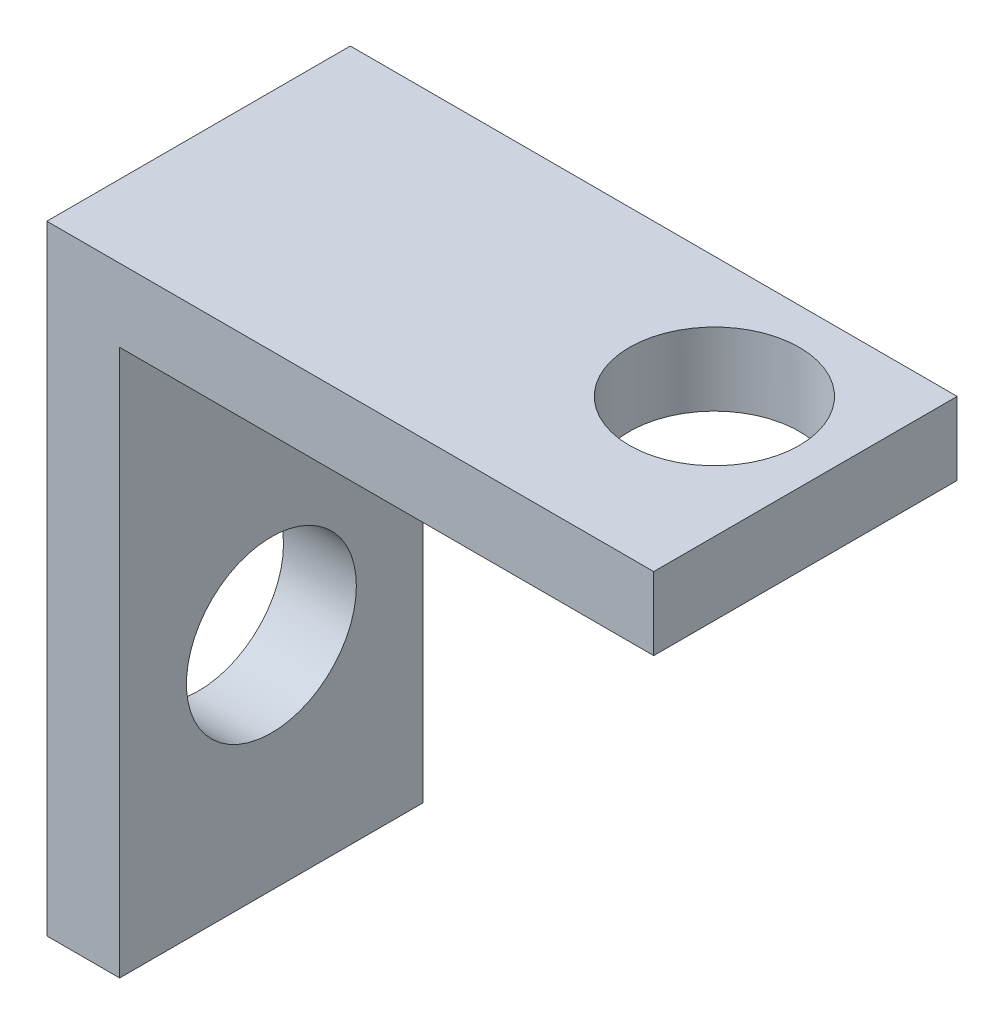
from build123d import *

# Parameters (mm, degrees)
SKETCH1_W               = 40
SKETCH1_H               = 50
BOSS_EXTRUDE1_DEPTH     = 12
CUT_EXTRUDE1_DEPTH      = 35.190641995
CUT_EXTRUDE1_DEPTH_BACK = 35.190641995
SKETCH2_R               = 14
MOVE_FACE2_BY           = 60
SKETCH3_W               = 12
SKETCH3_H               = 50
BOSS_EXTRUDE2_DEPTH     = 90
CUT_EXTRUDE2_DEPTH      = 129.33160172
CUT_EXTRUDE2_DEPTH_BACK = 129.33160172
SKETCH4_R               = 14


with BuildPart() as part:
    # Sketch1 → Boss-Extrude1 (new body)
    with BuildSketch(Plane(origin=(0, 0, 0), x_dir=(1, 0, 0), z_dir=(0, 1, 0))):
        Rectangle(SKETCH1_W, SKETCH1_H)
    extrude(amount=BOSS_EXTRUDE1_DEPTH)

    # Sketch2 → Cut-Extrude1 (cut, two sides: drawn at the far end of the back side and taken through both)
    with BuildSketch(Plane(origin=(0, 12, 0), x_dir=(1, 0, 0), z_dir=(0, 1, 0)).offset(-CUT_EXTRUDE1_DEPTH_BACK)):
        with Locations(Location((0, 5, 0), (0, 0, 270))):
            Circle(SKETCH2_R)
    extrude(amount=CUT_EXTRUDE1_DEPTH + CUT_EXTRUDE1_DEPTH_BACK, mode=Mode.SUBTRACT)

    # Move Face2: a face moved outward by 60.0
    extrude(part.faces().sort_by_distance((-20, 6, 0))[0], amount=MOVE_FACE2_BY, dir=(-1, 0, 0))

    # Sketch3 → Boss-Extrude2 (add)
    with BuildSketch(Plane(origin=(0, 0, 0), x_dir=(1, 0, 0), z_dir=(0, 1, 0))):
        with Locations((-74, 0)):
            Rectangle(SKETCH3_W, SKETCH3_H)
    extrude(amount=-BOSS_EXTRUDE2_DEPTH)

    # Sketch4 → Cut-Extrude2 (cut, two sides: drawn at the far end of the back side and taken through both)
    with BuildSketch(Plane(origin=(-68, 0, 0), x_dir=(0, 0, -1), z_dir=(1, 0, 0)).offset(-CUT_EXTRUDE2_DEPTH_BACK)):
        with Locations((0, -53.54)):
            Circle(SKETCH4_R)
    extrude(amount=CUT_EXTRUDE2_DEPTH + CUT_EXTRUDE2_DEPTH_BACK, mode=Mode.SUBTRACT)


solid = part.part
